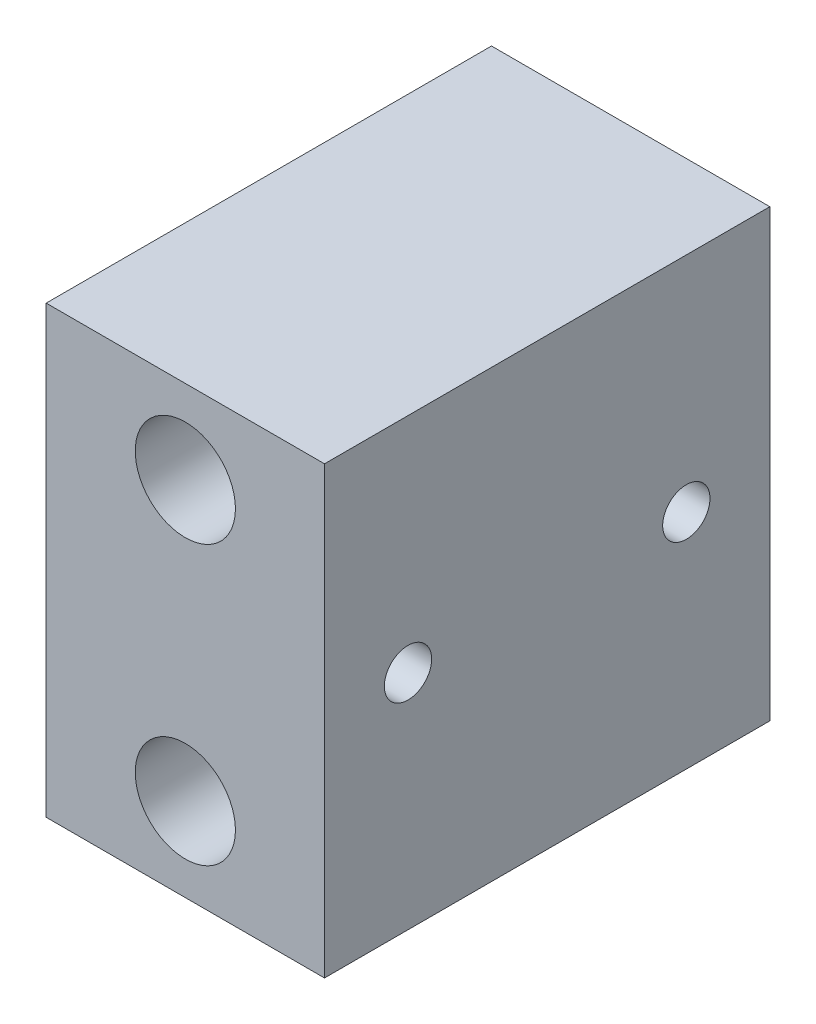
from build123d import *

# Parameters (mm, degrees)
SKETCH_1_W                = 80
SKETCH_1_H                = 80
EXTRUDE_1_DEPTH           = 50
HOLE_WIZARD_1_D           = 11
HOLE_WIZARD_1_CBORE_D     = 18
HOLE_WIZARD_1_CBORE_DEPTH = 30
HOLE_WIZARD_M10_1_D       = 8.5


with BuildPart() as part:
    # 草图1 → 凸台-拉伸1 (new body)
    with BuildSketch(Plane(origin=(0, 0, 0), x_dir=(0, 0, -1), z_dir=(1, 0, 0))):
        Rectangle(SKETCH_1_W, SKETCH_1_H)
    extrude(amount=EXTRUDE_1_DEPTH)

    # 打孔尺寸(%根据)内六角圆柱头螺钉的类型1 (through all)
    with Locations(Plane.XY.offset(40)):
        with Locations((25, 25), (25, -25)):
            CounterBoreHole(HOLE_WIZARD_1_D / 2, HOLE_WIZARD_1_CBORE_D / 2, HOLE_WIZARD_1_CBORE_DEPTH)

    # M10 螺纹孔1 (through all)
    with Locations(Plane(origin=(50, 0, 0), x_dir=(0, 0, -1), z_dir=(1, 0, 0))):
        with Locations((25, 0), (-25, 0)):
            Hole(HOLE_WIZARD_M10_1_D / 2)


solid = part.part
